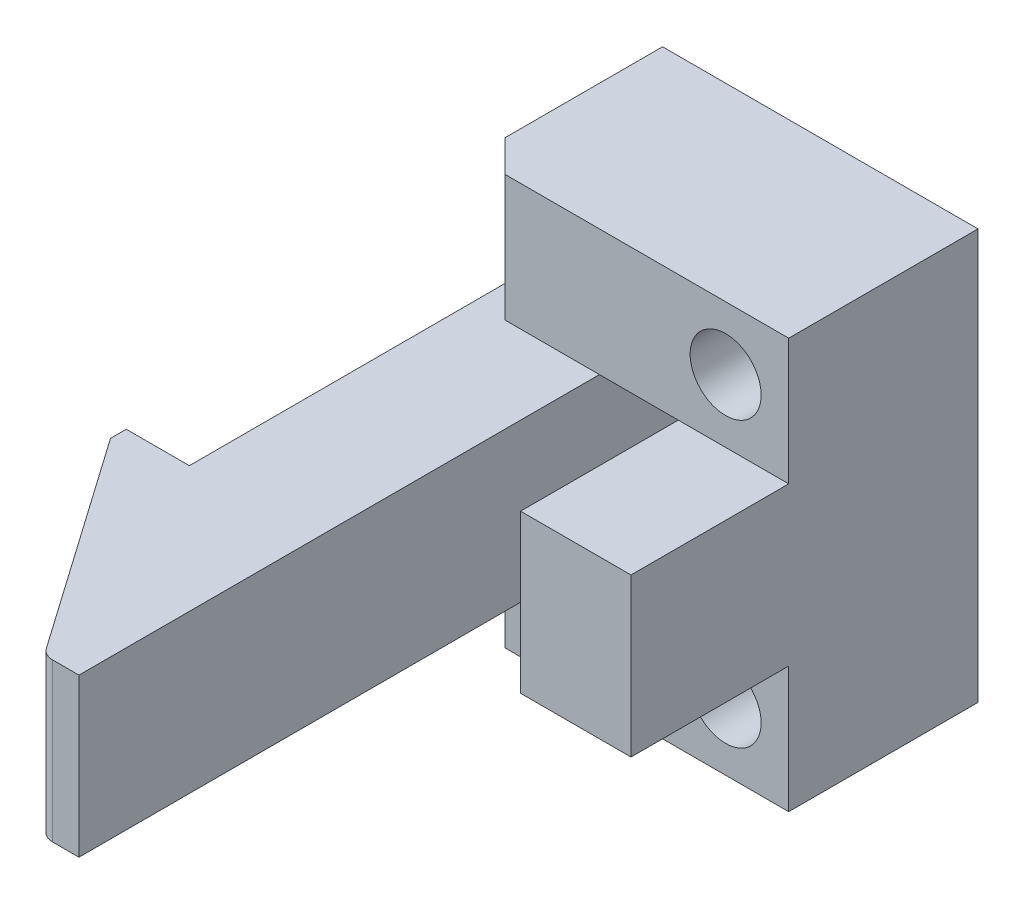
SolidWorks part; units mm, degrees
material "45 "
ref_plane "Front Plane" through (0, 0, 0) normal (0, 0, 1) x (1, 0, 0)
ref_plane "Top Plane" through (0, 0, 0) normal (0, 1, 0) x (1, 0, 0)
ref_plane "Right Plane" through (0, 0, 0) normal (1, 0, 0) x (0, 0, -1)
sketch "Sketch1" plane through (0, 0, 0) normal (0, 0, 1) x (1, 0, 0)
  line L1 (10, -13) -> (-10, -13)
  line L2 (10, -13) -> (10, 13)
  line L3 (10, 13) -> (-10, 13)
  line L4 (-10, -13) -> (-10, 13)
  line L5 (10, -13) -> (-10, 13) construction
  line L6 (10, 13) -> (-10, -13) construction
  point P0 (0, 0)
  dimension "D1" = 20
  dimension "D2" = 26
extrude "Boss-Extrude1" add sketch "Sketch1" along normal blind 12
sketch "Sketch2" plane through (0, 0, 12) normal (0, 0, 1) x (1, 0, 0)
  line L0 (10, -13) -> (10, 13) construction
  line L1 (10, 13) -> (-10, 13) construction
  line L2 (-10, -13) -> (10, -13) construction
  circle A0 centre (6, 9) radius 2.25
  circle A1 centre (6, -9) radius 2.25
  dimension "D1" = 4
  dimension "D2" = 18
  dimension "D4" = 4
  dimension "D5" = 4.5
  dimension "D3" = 4
extrude "Cut-Extrude1" cut sketch "Sketch2" against normal up to next
sketch "Sketch3" plane through (0, 0, 12) normal (0, 0, 1) x (1, 0, 0)
  line L0 (10, -13) -> (10, 13) construction
  line L1 (10, 5) -> (3, 5)
  line L2 (10, 5) -> (10, -5)
  line L3 (10, -5) -> (3, -5)
  line L4 (3, 5) -> (3, -5)
  line L5 (10, 13) -> (-10, 13) construction
  line L6 (-10, -13) -> (10, -13) construction
  dimension "D1" = 10
  dimension "D2" = 7
  dimension "D3" = 8
  dimension "D4" = 8
extrude "Boss-Extrude2" add sketch "Sketch3" along normal blind 10
sketch "Sketch4" plane through (0, 0, 12) normal (0, 0, 1) x (1, 0, 0)
  line L0 (-10, 13) -> (-10, -13) construction
  line L1 (3, 5) -> (-10, 5)
  line L2 (3, 5) -> (3, -5)
  line L3 (3, -5) -> (-10, -5)
  line L4 (-10, 5) -> (-10, -5)
  line L5 (3, -5) -> (10, -5) construction
extrude "Cut-Extrude2" cut sketch "Sketch4" against normal up to next
sketch "Sketch5" plane through (0, 0, 0) normal (0, 1, 0) x (1, 0, 0)
  line L0 (-10, -2) -> (-10, -30)
  line L1 (-10, -30) -> (-14, -30)
  line L2 (-14, -30) -> (-14, -31)
  line L3 (-14, -31) -> (-4.1971, -45)
  line L4 (-4.1971, -45) -> (-2, -45)
  line L5 (-2, -45) -> (-2, -2)
  line L6 (-2, -2) -> (-10, -2)
  line L7 (-10, -12) -> (-10, 0) construction
  line L8 (-10, 0) -> (3, 0) construction
  line L9 (-10, 0) -> (10, 0) construction
  dimension "D1" = 8
  dimension "D2" = 2
  dimension "D3" = 4
  dimension "D4" = 35
  dimension "D5" = 1
  dimension "D6" = 45
  dimension "D7" = 4
  dimension "D8" = 30
extrude "Boss-Extrude3" add sketch "Sketch5" along normal blind 5 and the other way blind 5 separate body
chamfer "Chamfer1" distance 2 angle 45 2 edges at (-10, -9, 12) (-10, 9, 12)
fillet "Fillet1" radius 1 1 edges at (-4.1971, 0, 45)
